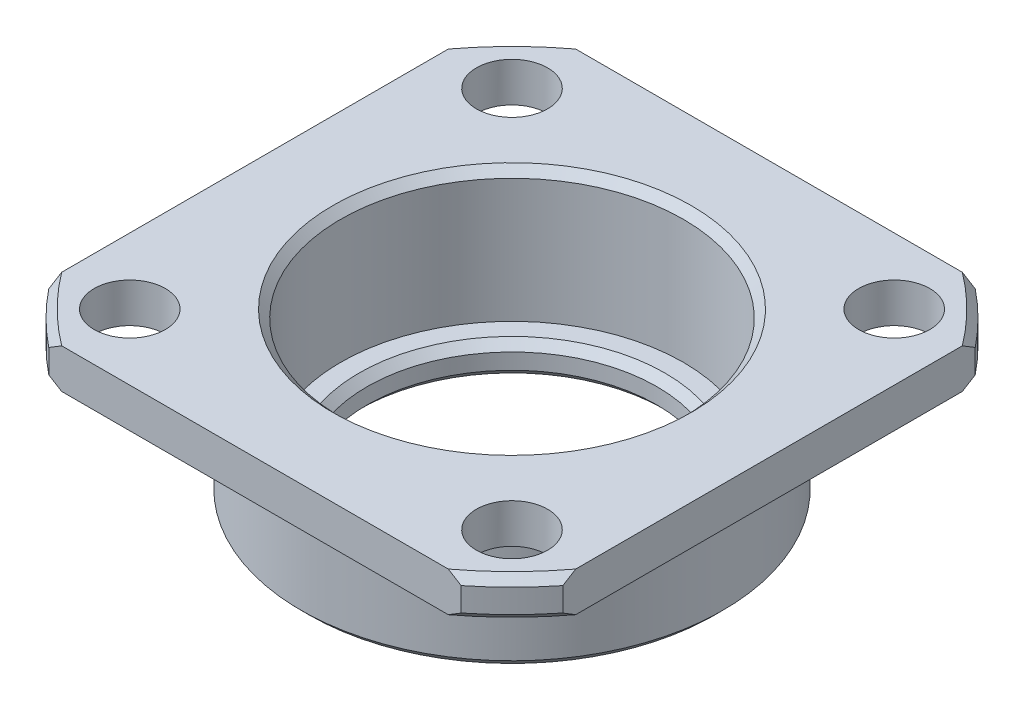
SolidWorks part; units mm, degrees
material "SUS 303"
ref_plane "Front Plane" through (0, 0, 0) normal (0, 0, 1) x (1, 0, 0)
ref_plane "Top Plane" through (0, 0, 0) normal (0, 1, 0) x (1, 0, 0)
ref_plane "Right Plane" through (0, 0, 0) normal (1, 0, 0) x (0, 0, -1)
sketch "Sketch1" plane through (0, 0, 0) normal (0, 0, 1) x (1, 0, 0)
  line L0 (5.8, 0) -> (7.7, 0)
  line L1 (8, 0.3) -> (8, 4.7)
  line L2 (8, 4.7) -> (12.2, 4.7)
  line L3 (12.5, 5) -> (12.5, 5.9)
  line L4 (12.2, 6.2) -> (6.8, 6.2)
  line L5 (6.5, 5.9) -> (6.5, 1.2)
  line L6 (6.5, 1.2) -> (5.8, 1.2)
  line L7 (5.5, 0.9) -> (5.5, 0.3)
  line L8 (0, 0) -> (0, 4.1352) construction
  line L9 (5.8, 1.2) -> (5.5, 0.9)
  line L10 (5.5, 0.3) -> (5.8, 0)
  line L11 (7.7, 0) -> (8, 0.3)
  line L12 (6.8, 6.2) -> (6.5, 5.9)
  line L13 (12.5, 5.9) -> (12.2, 6.2)
  line L14 (12.2, 4.7) -> (12.5, 5)
  point P0 (5.5, 0)
  point P1 (8, 0)
  point P5 (12.5, 4.7)
  point P6 (12.5, 6.2)
  point P7 (6.5, 6.2)
  point P9 (5.5, 1.2)
  dimension "D1" = 13
  dimension "D2" = 16
  dimension "D3" = 25
  dimension "D4" = 1.2
  dimension "D5" = 1.5
  dimension "D6" = 5
  dimension "D7" = 1
revolve "Revolve1" add sketch "Sketch1" angle 360 about L8
sketch "Sketch2" plane through (0, 6.2, 0) normal (0, 1, 0) x (1, 0, 0)
  line L1 (-9.75, 9.75) -> (9.75, 9.75)
  line L2 (-9.75, 9.75) -> (-9.75, -9.75)
  line L3 (-9.75, -9.75) -> (9.75, -9.75)
  line L4 (9.75, 9.75) -> (9.75, -9.75)
  line L5 (-9.75, 9.75) -> (9.75, -9.75) construction
  line L6 (-9.75, -9.75) -> (9.75, 9.75) construction
  point P0 (0, 0)
  dimension "D1" = 19.5
  dimension "D2" = 19.5
extrude "Cut-Extrude1" cut sketch "Sketch2" against normal through all flip side to cut
sketch "Sketch3" plane through (0, 6.2, 0) normal (0, 1, 0) x (1, 0, 0)
  line L0 (-7.25, 7.25) -> (0, 0) construction
  line L1 (0, 0) -> (0, 3.1835) construction
  line L2 (0, 0) -> (2.3301, 0) construction
  circle A0 centre (-7.25, 7.25) radius 1.35
  circle A1 centre (7.25, 7.25) radius 1.35
  circle A2 centre (7.25, -7.25) radius 1.35
  circle A3 centre (-7.25, -7.25) radius 1.35
  dimension "D3" = 2.7
  dimension "D1" = 45
  dimension "D2" = 7.25
extrude "Cut-Extrude2" cut sketch "Sketch3" against normal blind 10
